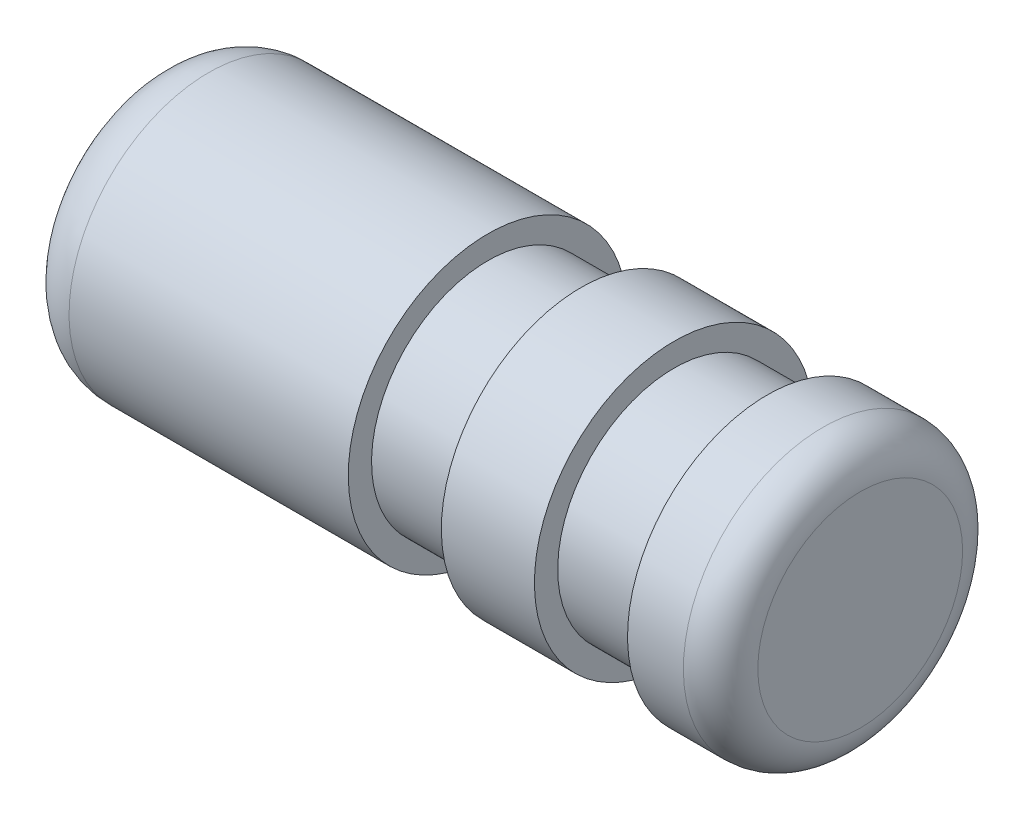
from build123d import *


with BuildPart() as part:
    # 草图1 → 旋转1 (revolve)
    with BuildSketch(Plane.XY, mode=Mode.PRIVATE) as revolve_1_sk:
        with BuildLine():
            Line((1.35, 0.75), (1.35, 0.625))
            Line((1.35, 0.625), (0.85, 0.625))
            Line((0.85, 0.625), (0.85, 0.75))
            Line((0.85, 0.75), (0.35, 0.75))
            Line((0.35, 0.75), (0.35, 0.625))
            Line((0.35, 0.625), (-0.15, 0.625))
            Line((-0.15, 0.625), (-0.15, 0.75))
            Line((-0.15, 0.75), (-1.65, 0.75))
            ThreePointArc((-1.65, 0.75), (-1.862132034, 0.662132034), (-1.95, 0.45))
            Line((-1.95, 0.45), (-1.95, 0))
            Line((-1.95, 0), (1.85, 0))
            Line((1.85, 0), (1.85, 0.55))
            ThreePointArc((1.85, 0.55), (1.791421356, 0.691421356), (1.65, 0.75))
            Line((1.65, 0.75), (1.35, 0.75))
        make_face()
    revolve(revolve_1_sk.sketch.rotate(Axis((-2.528803116, 0, 0), (1, 0, 0)), 180), axis=Axis((-2.528803116, 0, 0), (1, 0, 0)))


solid = part.part
